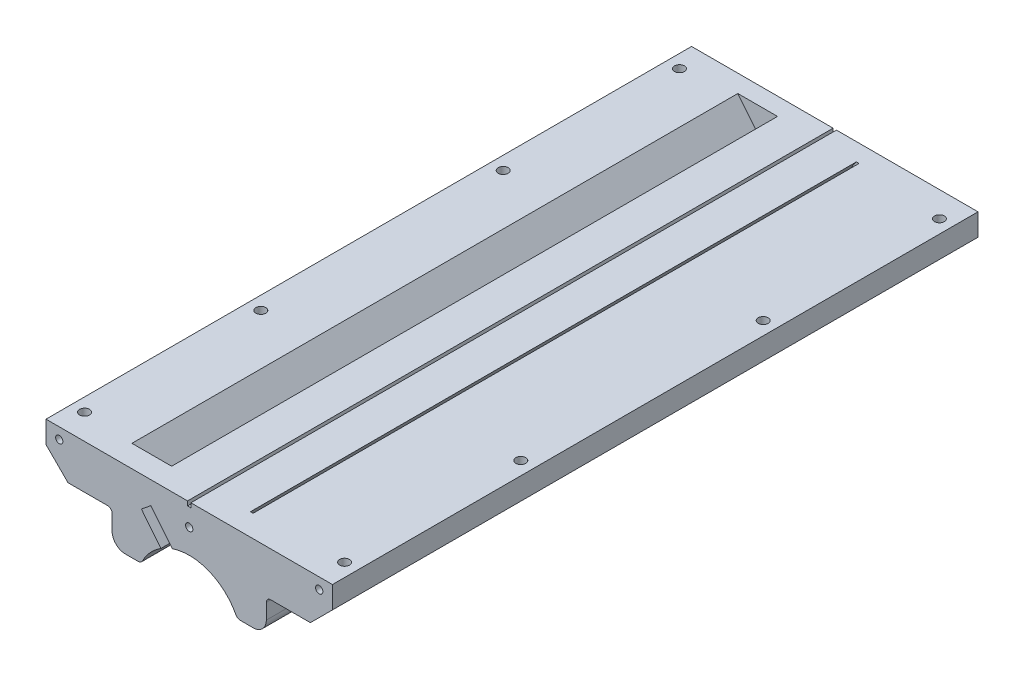
from build123d import *

# Parameters (mm, degrees)
SKETCH1_W                                            = 130
SKETCH1_H                                            = 35
BOSS_EXTRUDE1_DEPTH                                  = 146.5
SKETCH3_R                                            = 24
CUT_EXTRUDE2_DEPTH                                   = 301.633082012
SKETCH7_W                                            = 30
SKETCH7_H                                            = 293
CUT_EXTRUDE5_DEPTH                                   = 15
FILLET1_R                                            = 6
CHAMFER1_SIZE                                        = 10
FILLET2_R                                            = 2
CUT_EXTRUDE6_DEPTH                                   = 275
CUT_EXTRUDE8_DEPTH                                   = 301.633082012
FILLET3_R                                            = 2
M4_TAPPED_HOLE1_AT_2_COUNT                           = 2
M4_TAPPED_HOLE1_AT_2_PITCH                           = 59.211485372
M4_TAPPED_HOLE1_AT_3_COUNT                           = 2
M4_TAPPED_HOLE1_AT_3_PITCH                           = 59.211485372
SKETCH15_W                                           = 1.5
SKETCH15_H                                           = 4
CUT_EXTRUDE9_DEPTH                                   = 301.633082012
HOLE_SIZE_PER_SOCKET_HEAD_CAP_SCREW_TYPE_D           = 4.5
HOLE_SIZE_PER_SOCKET_HEAD_CAP_SCREW_TYPE_CBORE_D     = 8
HOLE_SIZE_PER_SOCKET_HEAD_CAP_SCREW_TYPE_CBORE_DEPTH = 15
LPATTERN1_COUNT                                      = 2
LPATTERN1_PITCH                                      = 80
MIRROR2_COPY_1_D                                     = 4.5
MIRROR2_COPY_1_CBORE_D                               = 8
MIRROR2_COPY_1_CBORE_DEPTH                           = 15


with BuildPart() as part:
    # Sketch1 → Boss-Extrude1 (new, symmetric)
    with BuildSketch(Plane.XY):
        Rectangle(SKETCH1_W, SKETCH1_H)
    extrude(amount=BOSS_EXTRUDE1_DEPTH, both=True)

    # Sketch3 → Cut-Extrude2 (cut, through all)
    with BuildSketch(Plane.XY.offset(146.5)):
        with Locations((0, -27.5)):
            Circle(SKETCH3_R)
    extrude(amount=-CUT_EXTRUDE2_DEPTH, mode=Mode.SUBTRACT)

    # Sketch7 → Cut-Extrude5 (cut)
    with BuildSketch(Plane.XZ.offset(17.5)):
        with Locations((-50, 0)):
            Rectangle(SKETCH7_W, SKETCH7_H)
        with Locations((50, 0)):
            Rectangle(SKETCH7_W, SKETCH7_H)
    extrude(amount=-CUT_EXTRUDE5_DEPTH, mode=Mode.SUBTRACT)

    # Fillet1
    fillet1_edges = [part.edges().sort_by_distance(p)[0] for p in [
        (-35, -17.5, 0),
        (35, -17.5, 0),
    ]]
    fillet(fillet1_edges, radius=FILLET1_R)

    # Chamfer1
    chamfer1_edges = [part.edges().sort_by_distance(p)[0] for p in [
        (-65, -2.5, 0),
        (65, -2.5, 0),
    ]]
    chamfer(chamfer1_edges, length=CHAMFER1_SIZE)

    # Fillet2
    fillet2_edges = [part.edges().sort_by_distance(p)[0] for p in [
        (-35, -2.5, 0),
        (35, -2.5, 0),
    ]]
    fillet(fillet2_edges, radius=FILLET2_R)

    # Sketch8 → Cut-Extrude6 (cut)
    with BuildSketch(Plane.XY.offset(136.5)):
        Polygon((-36, 17.5), (-25.11995654, 26.310485475), (-0.29024799, -4.351651011), (-11.170291451, -13.162136485), align=None)
        Polygon((18.180847956, 18.073576436), (19, 17.5), (3.82412996, -4.173388548), (3.004977916, -3.599812112), align=None)
    extrude(amount=-CUT_EXTRUDE6_DEPTH, mode=Mode.SUBTRACT)

    # Sketch10 → Cut-Extrude8 (cut, through all)
    with BuildSketch(Plane.XY.offset(146.5)):
        Polygon((-21.705399374, 3.820177656), (-17.431096586, 7.281439807), (-4.844688765, -8.261479422), (-9.118991553, -11.722741573), align=None)
    extrude(amount=-CUT_EXTRUDE8_DEPTH, mode=Mode.SUBTRACT)

    # Fillet3
    fillet3_edges = [part.edges().sort_by_distance(p)[0] for p in [
        (-21.817424229, -17.5, 0),
        (21.817424229, -17.5, 0),
    ]]
    fillet(fillet3_edges, radius=FILLET3_R)

    # Sketch11 → M4 Tapped Hole1 (revolve, cut)
    with BuildSketch(Plane(origin=(0, 7.5, 146.5), x_dir=(0, -1, 0), z_dir=(1, 0, 0))):
        Polygon((0, 0), (0, 12.491420021), (1.65, 11.5), (1.65, 0), align=None)
    m4_tapped_hole1 = revolve(axis=Axis((0, 7.5, 152.85), (0, 0, -1)), mode=Mode.SUBTRACT)

    # M4 Tapped Hole1 at 2: M4 Tapped Hole1 ×2
    with Locations(*[Vector(0.9964283048969313, 0.08444307668618053, 0) * (i * M4_TAPPED_HOLE1_AT_2_PITCH) for i in range(1, M4_TAPPED_HOLE1_AT_2_COUNT)]):
        add(m4_tapped_hole1, mode=Mode.SUBTRACT)

    # M4 Tapped Hole1 at 3: M4 Tapped Hole1 ×2
    with Locations(*[Vector(-0.9964283048969313, 0.08444307668618053, 0) * (i * M4_TAPPED_HOLE1_AT_3_PITCH) for i in range(1, M4_TAPPED_HOLE1_AT_3_COUNT)]):
        add(m4_tapped_hole1, mode=Mode.SUBTRACT)

    # Mirror1: M4 Tapped Hole1 across plane
    add(m4_tapped_hole1.mirror(Plane.XY), mode=Mode.SUBTRACT)

    # Mirror1 copy 1 sketch → Mirror1 copy 1 (revolve, cut)
    with BuildSketch(Plane(origin=(59, 12.5, -146.5), x_dir=(0, -1, 0), z_dir=(1, 0, 0))):
        Polygon((0, 0), (0, -12.491420021), (1.65, -11.5), (1.65, 0), align=None)
    revolve(axis=Axis((59, 12.5, -152.85), (0, 0, -1)), mode=Mode.SUBTRACT)

    # Mirror1 copy 2 sketch → Mirror1 copy 2 (revolve, cut)
    with BuildSketch(Plane(origin=(-59, 12.5, -146.5), x_dir=(0, -1, 0), z_dir=(1, 0, 0))):
        Polygon((0, 0), (0, -12.491420021), (1.65, -11.5), (1.65, 0), align=None)
    revolve(axis=Axis((-59, 12.5, -152.85), (0, 0, -1)), mode=Mode.SUBTRACT)

    # Sketch15 → Cut-Extrude9 (cut, through all)
    with BuildSketch(Plane(origin=(0, 0, -146.5), x_dir=(-1, 0, 0), z_dir=(0, 0, -1))):
        with Locations((0, 17.5)):
            Rectangle(SKETCH15_W, SKETCH15_H)
    extrude(amount=-CUT_EXTRUDE9_DEPTH, mode=Mode.SUBTRACT)

    # Hole size per socket head cap screw type 1 (through all)
    with Locations(Plane(origin=(0, -2.5, 0), x_dir=(-1, 0, 0), z_dir=(0, -1, 0))):
        with Locations((59, -135), (-59, -135)):
            hole_size_per_socket_head_cap_screw_type = CounterBoreHole(HOLE_SIZE_PER_SOCKET_HEAD_CAP_SCREW_TYPE_D / 2, HOLE_SIZE_PER_SOCKET_HEAD_CAP_SCREW_TYPE_CBORE_D / 2, HOLE_SIZE_PER_SOCKET_HEAD_CAP_SCREW_TYPE_CBORE_DEPTH)

    # LPattern1: Hole size per socket head cap screw type 1 ×2
    with Locations(*[(0, 0, -i * LPATTERN1_PITCH) for i in range(1, LPATTERN1_COUNT)]):
        add(hole_size_per_socket_head_cap_screw_type, mode=Mode.SUBTRACT)

    # Mirror2: Hole size per socket head cap screw type 1 across plane
    add(hole_size_per_socket_head_cap_screw_type.mirror(Plane.XY), mode=Mode.SUBTRACT)

    # Mirror2 copy 1 (through all)
    with Locations(Plane(origin=(0, -2.5, 80), x_dir=(-1, 0, 0), z_dir=(0, -1, 0))):
        with Locations((59, 135), (-59, 135)):
            CounterBoreHole(MIRROR2_COPY_1_D / 2, MIRROR2_COPY_1_CBORE_D / 2, MIRROR2_COPY_1_CBORE_DEPTH)


solid = part.part
